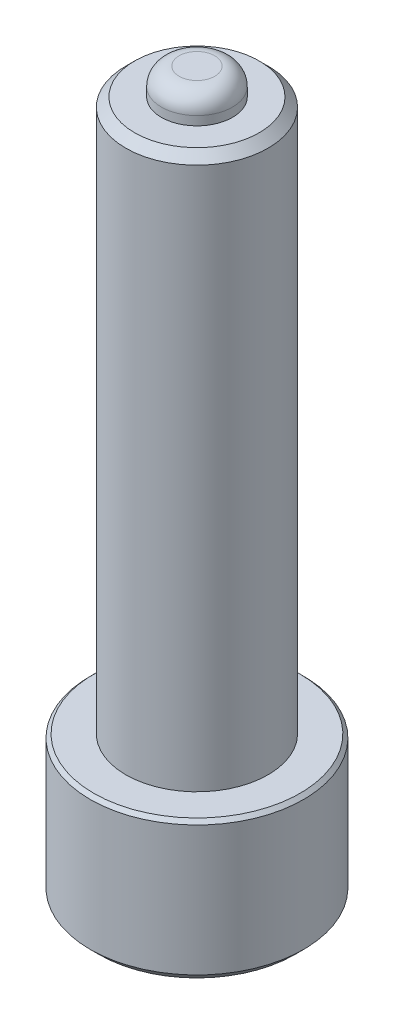
from build123d import *

# Parameters (mm, degrees)
SKETCH1_R           = 6
BOSS_EXTRUDE1_DEPTH = 4
SKETCH2_R           = 4
BOSS_EXTRUDE2_DEPTH = 31
SKETCH3_R           = 2
BOSS_EXTRUDE3_DEPTH = 1.5
CUT_EXTRUDE1_DEPTH  = 4
CHAMFER1_SIZE       = 0.5
CHAMFER2_SIZE       = 0.2
FILLET1_R           = 1


with BuildPart() as part:
    # Sketch1 → Boss-Extrude1 (new, symmetric)
    with BuildSketch(Plane(origin=(0, 0, 0), x_dir=(1, 0, 0), z_dir=(0, 1, 0))):
        with Locations(Location((0, 0, 0), (0, 0, 270))):
            Circle(SKETCH1_R)
    extrude(amount=BOSS_EXTRUDE1_DEPTH, both=True)

    # Sketch2 → Boss-Extrude2 (add)
    with BuildSketch(Plane(origin=(0, 4, 0), x_dir=(1, 0, 0), z_dir=(0, 1, 0))):
        with Locations(Location((0, 0, 0), (0, 0, 270))):
            Circle(SKETCH2_R)
    extrude(amount=BOSS_EXTRUDE2_DEPTH)

    # Sketch3 → Boss-Extrude3 (add)
    with BuildSketch(Plane(origin=(0, 35, 0), x_dir=(1, 0, 0), z_dir=(0, 1, 0))):
        with Locations(Location((0, 0, 0), (0, 0, 270))):
            Circle(SKETCH3_R)
    extrude(amount=BOSS_EXTRUDE3_DEPTH)

    # Sketch4 → Cut-Extrude1 (cut)
    with BuildSketch(Plane.XZ.offset(4)):
        Polygon((2.886751346, 0), (1.443375673, 2.5), (-1.443375673, 2.5), (-2.886751346, 0), (-1.443375673, -2.5), (1.443375673, -2.5), align=None)
    extrude(amount=-CUT_EXTRUDE1_DEPTH, mode=Mode.SUBTRACT)

    # Chamfer1
    chamfer1_edges = [part.edges().sort_by_distance(p)[0] for p in [
        (0, -4, -6),
        (0, 35, -4),
    ]]
    chamfer(chamfer1_edges, length=CHAMFER1_SIZE)

    # Chamfer2
    chamfer2_edges = [part.edges().sort_by_distance(p)[0] for p in [
        (0, 4, -6),
    ]]
    chamfer(chamfer2_edges, length=CHAMFER2_SIZE)

    # Fillet1
    fillet1_edges = [part.edges().sort_by_distance(p)[0] for p in [
        (0, 36.5, -2),
    ]]
    fillet(fillet1_edges, radius=FILLET1_R)

    # Sketch5 → Cut-Revolve1 (revolve, cut)
    with BuildSketch(Plane(origin=(0, 0, 0), x_dir=(0, 0, -1), z_dir=(1, 0, 0))):
        Polygon((2.5, 0), (0, 1.443375673), (0, 0), align=None)
    revolve(axis=Axis((0, 0, 0), (0, -1, 0)), mode=Mode.SUBTRACT)


solid = part.part
